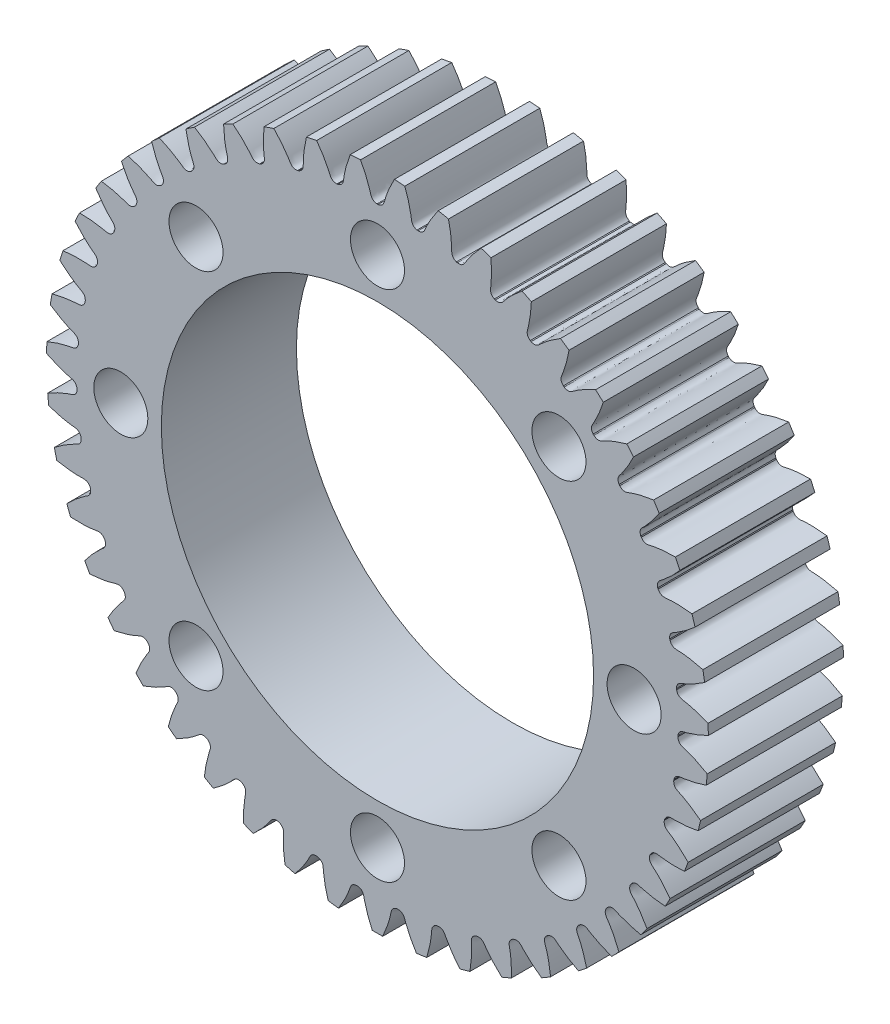
from build123d import *

# Parameters (mm, degrees)
SKETCH1_R           = 24.5
BOSS_EXTRUDE1_DEPTH = 10
CUT_EXTRUDE1_DEPTH  = 37.062445841
CIRPATTERN1_COUNT   = 47
SKETCH4_R           = 16
CUT_EXTRUDE2_DEPTH  = 37.059844592
SKETCH6_R           = 2
CUT_EXTRUDE4_DEPTH  = 8


with BuildPart() as part:
    # Sketch1 → Boss-Extrude1 (new body)
    with BuildSketch(Plane.XY):
        Circle(SKETCH1_R)
    extrude(amount=BOSS_EXTRUDE1_DEPTH)

    # Sketch2 → Cut-Extrude1 (cut, through all)
    with BuildSketch(Plane.XY):
        with BuildLine():
            ThreePointArc((0.038518442, 22.249966659), (0, 22.25), (-0.038518442, 22.249966659))
            add(Edge.make_bspline(
                [(-0.038518442, 22.249966659), (-0.439838637, 22.303150678), (-0.48799495, 22.603391057), (-0.586243717, 22.929649373), (-0.625168195, 23.05186917), (-0.669515449, 23.181570468), (-0.719428052, 23.318682703), (-0.775269468, 23.463002072), (-0.837331824, 23.614351724), (-0.905921639, 23.772534742), (-0.981334389, 23.937348083), (-1.063861599, 24.108578691), (-1.153788468, 24.286004809), (-1.251394242, 24.46939579), (-1.356951802, 24.658512352), (-1.470727476, 24.853106713), (-1.592980802, 25.052922763), (-1.723964297, 25.25769624), (-1.863923241, 25.467154908), (-2.013095459, 25.68101874), (-2.171711106, 25.899000114), (-2.339992461, 26.120804002), (-2.518153724, 26.346128176), (-2.706400814, 26.574663413), (-2.904931193, 26.806093707), (-3.113933597, 27.040096482), (-3.410816367, 27.359404461), (-3.643794283, 27.595186537), (-3.804218685, 27.751343297)],
                knots=[0, 0, 0, 0, 0.114836158, 0.132524592, 0.151521532, 0.171826979, 0.193440931, 0.216363391, 0.240594356, 0.266133828, 0.292981806, 0.321138291, 0.350603282, 0.381376779, 0.413458783, 0.446849293, 0.481548309, 0.517555832, 0.554871861, 0.593496396, 0.633429438, 0.674670986, 0.71722104, 0.761079601, 0.806246668, 0.852722241, 0.900506321, 1, 1, 1, 1], degree=3))
            ThreePointArc((-3.804218685, 27.751343297), (0, 28.010875291), (3.804218685, 27.751343297))
            add(Edge.make_bspline(
                [(0.038518442, 22.249966659), (0.439838637, 22.303150678), (0.48799495, 22.603391057), (0.586243717, 22.929649373), (0.625168195, 23.05186917), (0.669515449, 23.181570468), (0.719428052, 23.318682703), (0.775269468, 23.463002072), (0.837331824, 23.614351724), (0.905921639, 23.772534742), (0.981334389, 23.937348083), (1.063861599, 24.108578691), (1.153788468, 24.286004809), (1.251394242, 24.46939579), (1.356951802, 24.658512352), (1.470727476, 24.853106713), (1.592980802, 25.052922763), (1.723964297, 25.25769624), (1.863923241, 25.467154908), (2.013095459, 25.68101874), (2.171711106, 25.899000114), (2.339992461, 26.120804002), (2.518153724, 26.346128176), (2.706400814, 26.574663413), (2.904931193, 26.806093707), (3.113933597, 27.040096482), (3.410816367, 27.359404461), (3.643794283, 27.595186537), (3.804218685, 27.751343297)],
                knots=[0, 0, 0, 0, 0.114836158, 0.132524592, 0.151521532, 0.171826979, 0.193440931, 0.216363391, 0.240594356, 0.266133828, 0.292981806, 0.321138291, 0.350603282, 0.381376779, 0.413458783, 0.446849293, 0.481548309, 0.517555832, 0.554871861, 0.593496396, 0.633429438, 0.674670986, 0.71722104, 0.761079601, 0.806246668, 0.852722241, 0.900506321, 1, 1, 1, 1], degree=3))
        make_face()
    cut_extrude1 = extrude(amount=CUT_EXTRUDE1_DEPTH, mode=Mode.SUBTRACT)

    # CirPattern1: Cut-Extrude1 ×47 about axis
    cirpattern1_axis = Axis((0, 0, 10), (0, 0, -1))
    for i in range(1, CIRPATTERN1_COUNT):
        add(cut_extrude1.rotate(cirpattern1_axis, i * 360 / CIRPATTERN1_COUNT), mode=Mode.SUBTRACT)

    # Sketch4 → Cut-Extrude2 (cut, through all)
    with BuildSketch(Plane.XY.offset(10)):
        Circle(SKETCH4_R)
    extrude(amount=-CUT_EXTRUDE2_DEPTH, mode=Mode.SUBTRACT)

    # Sketch6 → Cut-Extrude4 (cut)
    with BuildSketch(Plane.XY.offset(10)):
        with Locations((0, 19)):
            Circle(SKETCH6_R)
        with Locations((13.435028843, 13.435028843)):
            Circle(SKETCH6_R)
        with Locations((19, 0)):
            Circle(SKETCH6_R)
        with Locations((13.435028843, -13.435028843)):
            Circle(SKETCH6_R)
        with Locations((0, -19)):
            Circle(SKETCH6_R)
        with Locations((-13.435028843, -13.435028843)):
            Circle(SKETCH6_R)
        with Locations((-19, 0)):
            Circle(SKETCH6_R)
        with Locations((-13.435028843, 13.435028843)):
            Circle(SKETCH6_R)
    extrude(amount=-CUT_EXTRUDE4_DEPTH, mode=Mode.SUBTRACT)


solid = part.part
